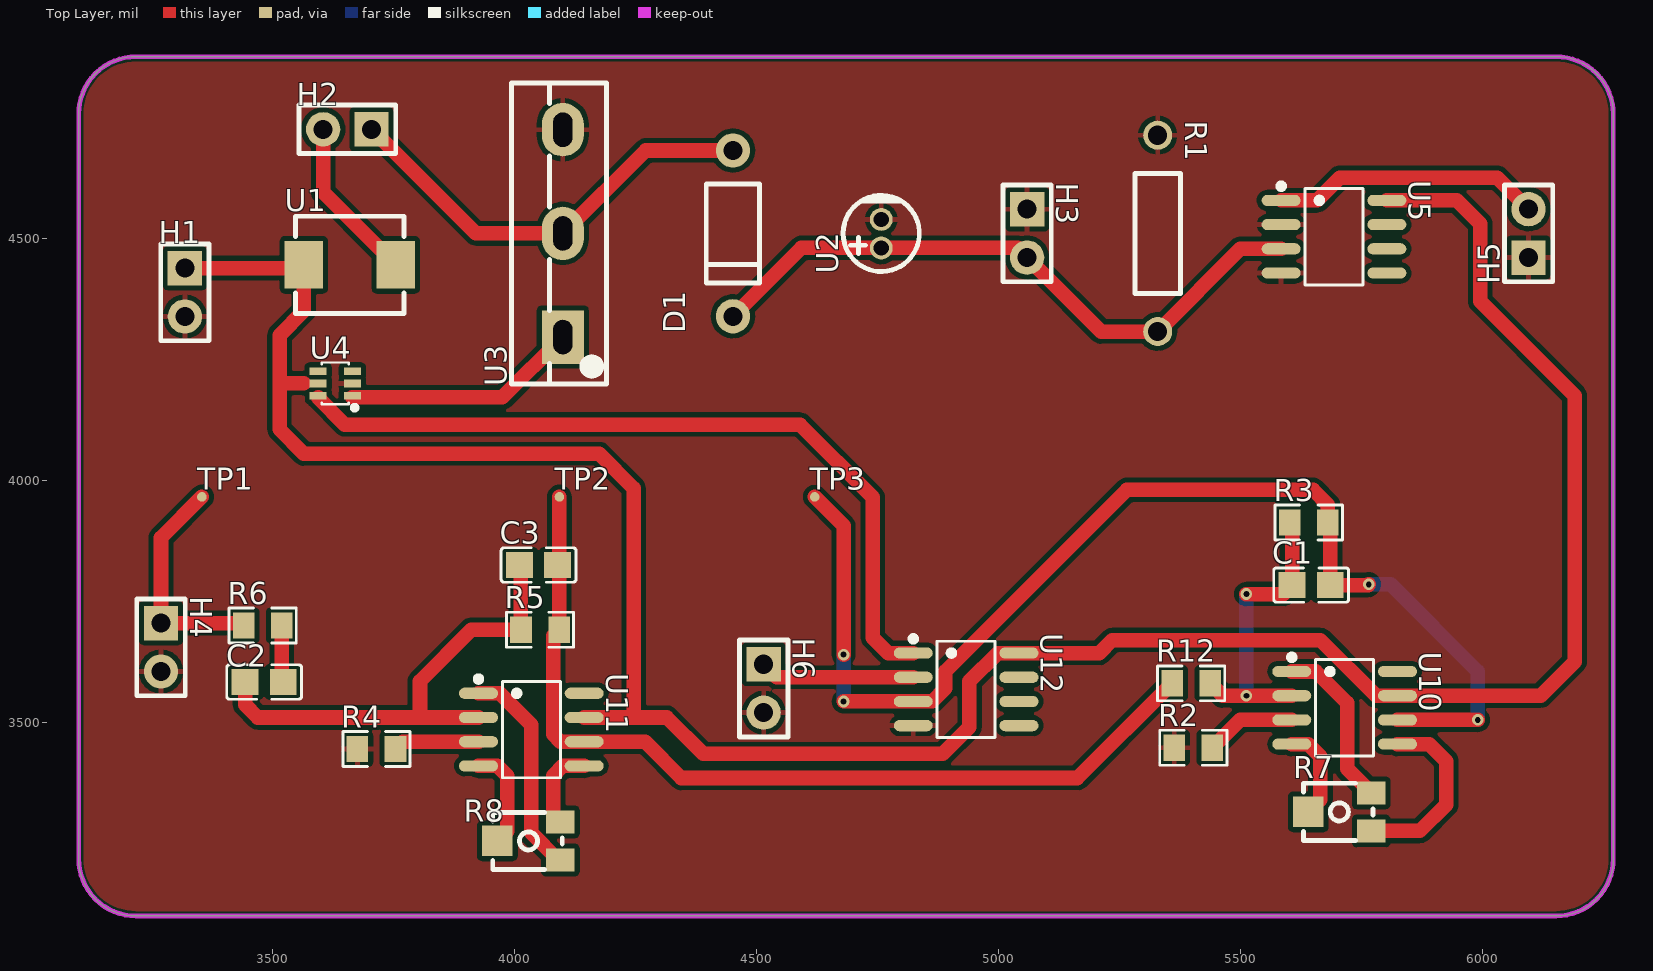
[diagram p0: Top Layer view]
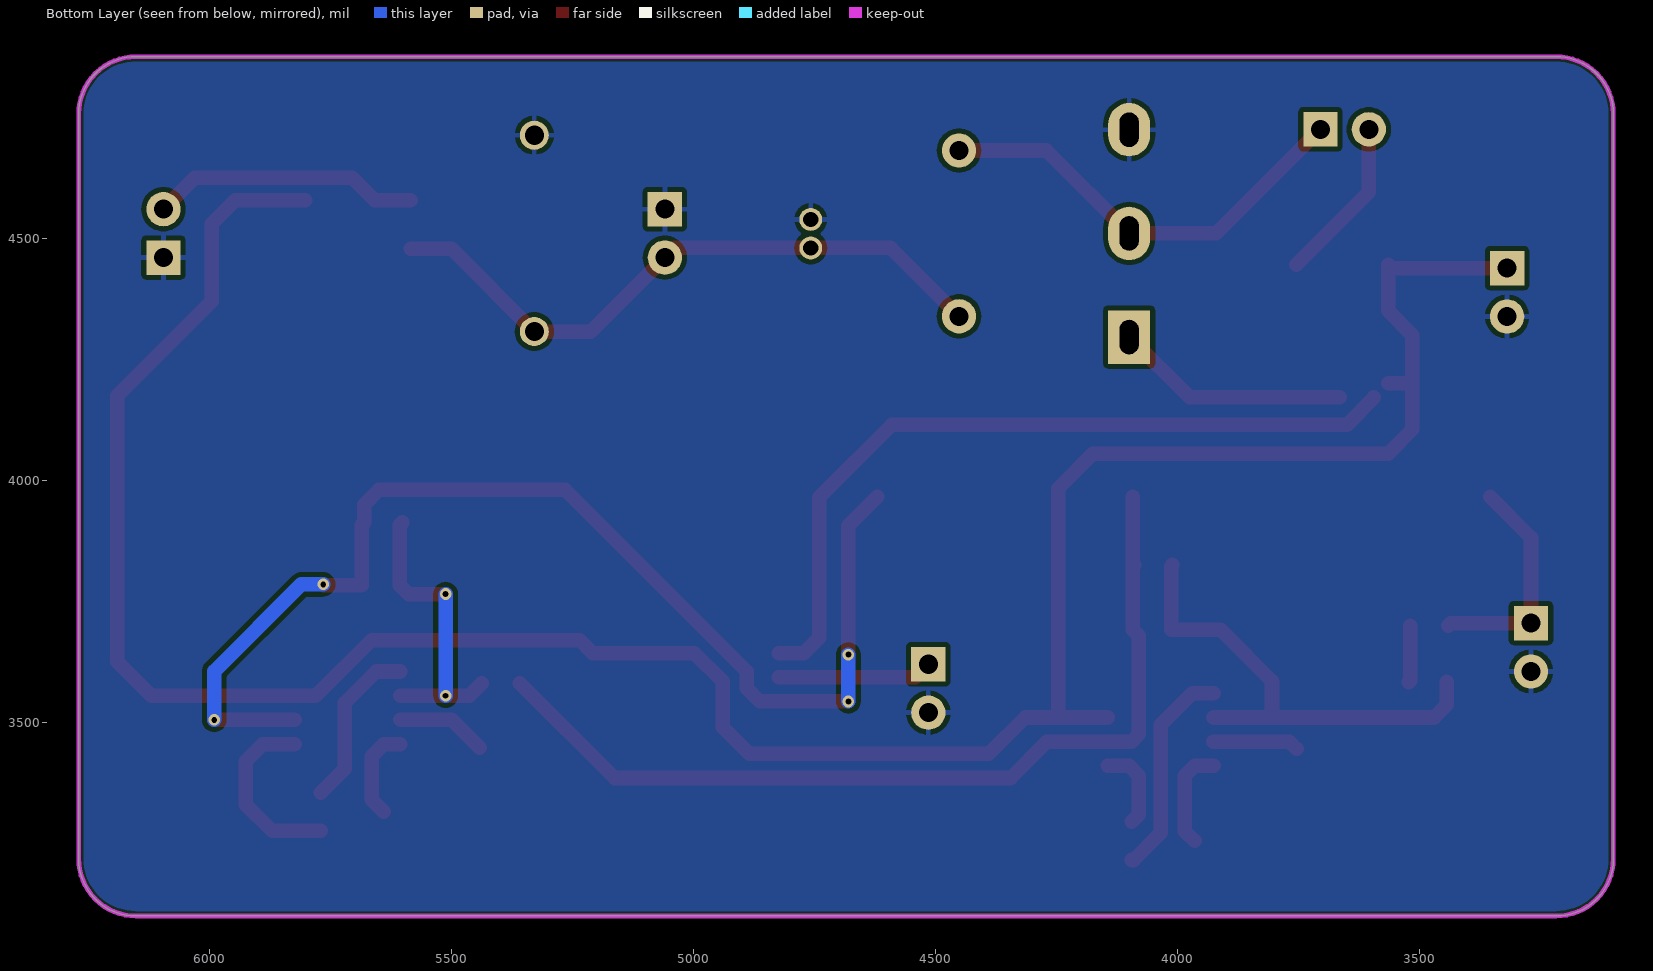
[diagram p1: Bottom Layer view, seen from below]
# Altium PCB MISC89040.pcbdoc
Units mil, origin at the board's own origin, x right, y up, seen from the top; angles counter-clockwise.
Board outline 3170 x 1775 mil, 2 copper layers (Top Layer, Bottom Layer), stack 62.206 mil thick; 30 components, 23 nets, 88 pads, 6 vias.

## Layer stack, top to bottom
Top Solder Mask Layer: solder mask 0.394, Dk 3.3
Top Layer: signal copper 1.379
Dielectric1: surface 59.449, FR4, Dk 4.5
Bottom Layer: signal copper 1.378
Bottom Solder Mask Layer: solder mask 0.394, Dk 3.3

## Board outline
3218.11,4875 ccw(c3218.11,4756.89) 3100,4756.89 3100,3218.11 ccw(c3218.11,3218.11) 3218.11,3100 6151.89,3100 ccw(c6151.89,3218.11) 6270,3218.11 6270,4756.89 ccw(c6151.89,4756.89) 6151.89,4875

## Design rules (kind name [scope] priority, off if disabled: settings)
BoardOutlineClearance copperThickness2oz_1 [All] p2 off: genericclearance=7.99 ignorepadtopadclearanceinfootprint=FALSE except(0: Arc-SplitContinuation Track-SplitContinuation SMDPad-SplitContinuation THPad-SplitContinuation Via-SplitContinuation Fill-SplitContinuation Region-SplitContinuation Poly-SplitContinuation Text-SplitContinuation Hole-SplitContinuation; 5.98: Arc-CutoutEdge Track-CutoutEdge SMDPad-CutoutEdge THPad-CutoutEdge Via-CutoutEdge Text-CutoutEdge; 6.9: Hole-OutlineEdge Hole-CutoutEdge; 10: Poly-OutlineEdge Poly-CutoutEdge; 11.81: Arc-OutlineEdge Track-OutlineEdge SMDPad-OutlineEdge THPad-OutlineEdge Via-OutlineEdge Fill-OutlineEdge Region-OutlineEdge Text-OutlineEdge Fill-CutoutEdge Region-CutoutEdge)
BoardOutlineClearance Plane_innerPlane_1 [All] p4 off: genericclearance=4.02 ignorepadtopadclearanceinfootprint=FALSE except(0: Arc-SplitContinuation Track-SplitContinuation SMDPad-SplitContinuation THPad-SplitContinuation Via-SplitContinuation Fill-SplitContinuation Region-SplitContinuation Poly-SplitContinuation Text-SplitContinuation Hole-SplitContinuation; 5.98: Arc-CutoutEdge Track-CutoutEdge SMDPad-CutoutEdge THPad-CutoutEdge Via-CutoutEdge Text-CutoutEdge; 6.9: Hole-OutlineEdge Hole-CutoutEdge; 10: Poly-OutlineEdge Poly-CutoutEdge; 11.81: Arc-OutlineEdge Track-OutlineEdge SMDPad-OutlineEdge THPad-OutlineEdge Via-OutlineEdge Fill-OutlineEdge Region-OutlineEdge Text-OutlineEdge Fill-CutoutEdge Region-CutoutEdge)
BoardOutlineClearance Copper_copperRegion_1 [All] p6 off: genericclearance=4.02 ignorepadtopadclearanceinfootprint=FALSE except(0: Arc-SplitContinuation Track-SplitContinuation SMDPad-SplitContinuation THPad-SplitContinuation Via-SplitContinuation Fill-SplitContinuation Region-SplitContinuation Poly-SplitContinuation Text-SplitContinuation Hole-SplitContinuation; 5.98: Arc-CutoutEdge Track-CutoutEdge SMDPad-CutoutEdge THPad-CutoutEdge Via-CutoutEdge Text-CutoutEdge; 6.9: Hole-OutlineEdge Hole-CutoutEdge; 10: Poly-OutlineEdge Poly-CutoutEdge; 11.81: Arc-OutlineEdge Track-OutlineEdge SMDPad-OutlineEdge THPad-OutlineEdge Via-OutlineEdge Fill-OutlineEdge Region-OutlineEdge Text-OutlineEdge Fill-CutoutEdge Region-CutoutEdge)
BoardOutlineClearance copperThickness1oz_1 [All] p8: genericclearance=4.02 ignorepadtopadclearanceinfootprint=FALSE except(0: Arc-SplitContinuation Track-SplitContinuation SMDPad-SplitContinuation THPad-SplitContinuation Via-SplitContinuation Fill-SplitContinuation Region-SplitContinuation Poly-SplitContinuation Text-SplitContinuation Hole-SplitContinuation; 5.98: Arc-CutoutEdge Track-CutoutEdge SMDPad-CutoutEdge THPad-CutoutEdge Via-CutoutEdge Text-CutoutEdge; 6.9: Hole-OutlineEdge Hole-CutoutEdge; 10: Poly-OutlineEdge Poly-CutoutEdge; 11.81: Arc-OutlineEdge Track-OutlineEdge SMDPad-OutlineEdge THPad-OutlineEdge Via-OutlineEdge Fill-OutlineEdge Region-OutlineEdge Text-OutlineEdge Fill-CutoutEdge Region-CutoutEdge)
Clearance copperThickness2oz [All] p1 off: gap=7.99 ignorepadtopadclearanceinfootprint=FALSE except(5.98: SMDPad-Track SMDPad-SMDPad THPad-Track SMDPad-THPad THPad-THPad Track-Via SMDPad-Via THPad-Via Via-Via Fill-SMDPad Region-SMDPad Fill-THPad Region-THPad Fill-Via Region-Via Fill-Fill Fill-Region Region-Region Arc-Track Arc-SMDPad Arc-THPad Arc-Via Fill-Arc Region-Arc Arc-Arc Text-Track SMDPad-Text Text-THPad Text-Via Fill-Text Region-Text Arc-Text Text-Text; 6.9: Hole-Track Hole-SMDPad Hole-THPad Hole-Via Fill-Hole Region-Hole Hole-Arc Hole-Text; 10: Poly-Track Poly-SMDPad Poly-THPad Poly-Via Poly-Fill Poly-Region Poly-Poly Poly-Arc Poly-Text Poly-Hole; 11.81: Fill-Track Region-Track)
Clearance Plane_innerPlane [All] p3 off: gap=4.02 ignorepadtopadclearanceinfootprint=FALSE except(5.98: SMDPad-Track SMDPad-SMDPad THPad-Track SMDPad-THPad THPad-THPad Track-Via SMDPad-Via THPad-Via Via-Via Fill-SMDPad Region-SMDPad Fill-THPad Region-THPad Fill-Via Region-Via Fill-Fill Fill-Region Region-Region Arc-Track Arc-SMDPad Arc-THPad Arc-Via Fill-Arc Region-Arc Arc-Arc Text-Track SMDPad-Text Text-THPad Text-Via Fill-Text Region-Text Arc-Text Text-Text; 6.9: Hole-Track Hole-SMDPad Hole-THPad Hole-Via Fill-Hole Region-Hole Hole-Arc Hole-Text; 10: Poly-Track Poly-SMDPad Poly-THPad Poly-Via Poly-Fill Poly-Region Poly-Poly Poly-Arc Poly-Text Poly-Hole; 11.81: Fill-Track Region-Track)
Clearance Copper_copperRegion [All] p5 off: gap=4.02 ignorepadtopadclearanceinfootprint=FALSE except(5.98: SMDPad-Track SMDPad-SMDPad THPad-Track SMDPad-THPad THPad-THPad Track-Via SMDPad-Via THPad-Via Via-Via Fill-SMDPad Region-SMDPad Fill-THPad Region-THPad Fill-Via Region-Via Fill-Fill Fill-Region Region-Region Arc-Track Arc-SMDPad Arc-THPad Arc-Via Fill-Arc Region-Arc Arc-Arc Text-Track SMDPad-Text Text-THPad Text-Via Fill-Text Region-Text Arc-Text Text-Text; 6.9: Hole-Track Hole-SMDPad Hole-THPad Hole-Via Fill-Hole Region-Hole Hole-Arc Hole-Text; 10: Poly-Track Poly-SMDPad Poly-THPad Poly-Via Poly-Fill Poly-Region Poly-Poly Poly-Arc Poly-Text Poly-Hole; 11.81: Fill-Track Region-Track)
Clearance copperThickness1oz [All] p7: gap=4.02 ignorepadtopadclearanceinfootprint=FALSE except(5.98: SMDPad-Track SMDPad-SMDPad THPad-Track SMDPad-THPad THPad-THPad Track-Via SMDPad-Via THPad-Via Via-Via Fill-SMDPad Region-SMDPad Fill-THPad Region-THPad Fill-Via Region-Via Fill-Fill Fill-Region Region-Region Arc-Track Arc-SMDPad Arc-THPad Arc-Via Fill-Arc Region-Arc Arc-Arc Text-Track SMDPad-Text Text-THPad Text-Via Fill-Text Region-Text Arc-Text Text-Text; 6.9: Hole-Track Hole-SMDPad Hole-THPad Hole-Via Fill-Hole Region-Hole Hole-Arc Hole-Text; 10: Poly-Track Poly-SMDPad Poly-THPad Poly-Via Poly-Fill Poly-Region Poly-Poly Poly-Arc Poly-Text Poly-Hole; 11.81: Fill-Track Region-Track)
DiffPairsRouting differentialPair [All] p1: maxlimit=6 minlimit=6 mostfreqgap=6 toplayer_minwidth=5 toplayer_prefwidth=10 toplayer_maxwidth=100 toplayer_mingap=6 toplayer_prefgap=6 toplayer_maxgap=6 bottomlayer_minwidth=5 bottomlayer_prefwidth=10 bottomlayer_maxwidth=100 bottomlayer_mingap=6 bottomlayer_prefgap=6 bottomlayer_maxgap=6 maxuncoupledlength=10
HoleToHoleClearance otherClearance [All] p1: gap=11.81 allowstackedmicrovias=TRUE
Length netLength [All] p1: minlimit=0 maxlimit=0
PasteMaskExpansion pasteMaskExpansion [All] p1: expansion=0
PlaneConnect innerPlane [All] p1: planeconnectstyle=Relief reliefexpansion=20 reliefentries=4 reliefconductorwidth=10 reliefairgap=10
PolygonConnect copperRegion [All] p1: connectstyle=Relief reliefconductorwidth=10 reliefentries=4 polygonreliefangle="90 Angle" airgapwidth=10 via.connectstyle=Relief via.reliefconductorwidth=10 via.reliefentries=4 via.polygonreliefangle="90 Angle" via.airgapwidth=10
RoutingVias viaSize [All] p1: holewidth=12.01 width=24.02 viastyle="Through Hole" minholewidth=11.81 minwidth=19.68 maxholewidth=248.03 maxwidth=393.7
SolderMaskExpansion solderMaskExpansion [IsVia] p1: expansion=-1000 istentingtop=TRUE
SolderMaskExpansion solderMaskExpansion [All] p2: expansion=2 istentingtop=FALSE
Width copperThickness2oz_2 [All] p1 off: maxlimit=100 minlimit=8 preferedwidth=10
Width copperThickness1oz_2 [All] p2: maxlimit=100 minlimit=5 preferedwidth=10

## Components (designator, comment, footprint, x,y, rotation, side; value= is the part's Value field where it differs from the comment)
C1 "100nF" C0805 5645.88,3783.59 r0 top
C2 "100nF" C0805 3483.1,3583.33 r180 top
C3 "1nF" C0805 4050,3825 r0 top
D1 "" DO_1N4007 4451.5,4510 r90 top
H1 "" HDR-TH_2P-P2.54-V-M-1 3319.36,4388.27 r270 top
H2 "" HDR-TH_2P-P2.54-V-M-1 3655,4725 r180 top
H3 "" HDR-TH_2P-P2.54-V-M-1 5059.14,4510 r270 top
H4 "" HDR-TH_2P-P2.54-V-M-1 3270,3655 r270 top
H5 "" HDR-TH_2P-P2.54-V-M-1 6095,4510 r90 top
H6 "" HDR-TH_2P-P2.54-V-M-1 4515,3570 r270 top
R1 "10kΩ" Res_1/4W 5328.9,4510 r270 top
R2 "10kΩ" R0805 5402.41,3447.47 r0 top
R3 "1MΩ" R0805 5640.88,3912.79 r0 top
R4 "10kΩ" R0805 3715,3445 r0 top
R5 "10kΩ" R0805 4052.94,3691.23 r0 top
R6 "100Ω" R0805 3480,3700 r0 top
R7 "100kΩ" RES-ADJ-SMD_VG039NCH 5705,3315 r0 top
R8 "100kΩ" RES-ADJ-SMD_VG039NCH 4030,3255 r0 top
R12 "10kΩ" R0805 5398.06,3580.66 r0 top
TP1 "" Test-Point-0.5mm 3354.36,3965.8 r0 top
TP2 "" Test-Point-0.5mm 4092.94,3965.8 r0 top
TP3 "" Test-Point-0.5mm 4620.38,3965.8 r0 top
U1 "Power inductor (SMD),CKST0502-10uH/M,10uH,±20%,3A,package 5.7mm*5.1mm*2.0mm,CENKER,RoHS" IND-SMD_L5.7-W5.1 3660,4445 r0 top
U2 "10uF" CAP-TH_BD4.0-P1.50-D0.8-FD 4757.84,4509.4 r90 top
U3 "HY5204" TO-247-3_L15.8-W5.0-P5.44-L-1 4100,4510 r90 top
U4 "SN74LVC2G04DCKR" SOT-363_L2.0-W1.3-P0.65-LS2.1-BR 3630,4200 r0 top
U5 "NE5532DR" SOIC-8_L4.9-W3.9-P1.27-LS6.0-BL 5693.07,4503.13 r270 top
U10 "UA741CDT" SOIC-8_L4.9-W3.9-P1.27-LS6.0-BL 5715,3530 r270 top
U11 "UA741CDT" SOIC-8_L4.9-W3.9-P1.27-LS6.0-BL 4035,3485 r270 top
U12 "NE5532DR" SOIC-8_L4.9-W3.9-P1.27-LS6.0-BL 4933.13,3568.13 r270 top

## Footprints (in the part's own frame and the unit in brackets; to place one, negate y for a bottom-side part, rotate by r counter-clockwise, add the part's x,y. Pads: shape width x height; smd on the part's side, far side on the other; paste and mask are expansions set on the pad)
C0805 [mm]
  rect 1.41x1.35 smd paste-100 mask+0.051: 1(-1,0) 2(1,0)
  silkscreen extent -1.96,-0.9 1.96,0.9
CAP-TH_BD4.0-P1.50-D0.8-FD [mm]
  round 1.2 hole 0.8: 1(-0.75,0) 2(0.75,0)
  silkscreen extent -1.98,-2 2.06,2
DO_1N4007 [mm]
  round 1.8 hole 1 paste+0 mask+0.051: 1(-4.35,0) 2(4.35,0)
  silkscreen extent -2.6,-1.4 2.6,1.4
HDR-TH_2P-P2.54-V-M-1 [mm]
  rect 1.8x1.8 hole 1: 1(-1.27,0)
  round 1.8 hole 1: 2(1.27,0)
  silkscreen extent -2.54,-1.27 2.54,1.27
IND-SMD_L5.7-W5.1 [mm]
  rect 2x2.5 smd paste+0 mask+0.05: 1(-2.413,0) 2(2.413,0)
  silkscreen extent -2.85,-2.55 2.85,2.55
R0805 [mm]
  rect 1.133x1.377 smd paste-100 mask+0.051: 1(-1,0) 2(1,0)
  silkscreen extent -1.76,-0.92 1.76,0.92
RES-ADJ-SMD_VG039NCH [mm]
  rect 1.5x1.2 smd: 1(1.65,-1) 3(1.65,1)
  rect 1.6x1.6 smd: 2(-1.65,0)
  silkscreen extent -1.9,-1.5 1.75,1.5
Res_1/4W [mil]
  round 60 hole 39.37 paste+0 mask+2: 1(-202.76,0) 2(202.76,0)
  silkscreen extent -124,-47 124,47
SOIC-8_L4.9-W3.9-P1.27-LS6.0-BL [mm]
  oval 0.588x2.045 smd: 1(-1.905,-2.772) 2(-0.635,-2.772) 3(0.635,-2.772) 4(1.905,-2.772) 5(1.905,2.772) 6(0.635,2.772) 7(-0.635,2.772) 8(-1.905,2.772)
  silkscreen extent -2.8,-2.92 2.53,1.52
SOT-363_L2.0-W1.3-P0.65-LS2.1-BR [mm]
  rect 0.9x0.4 smd: 1(0.9,-0.65) 2(0.9,0) 3(0.9,0.65) 4(-0.9,0.65) 5(-0.9,0) 6(-0.9,-0.65)
  silkscreen extent -0.7,-1.4 1.14,1.1
Test-Point-0.5mm [mm]
  round 0.5 smd: 1(0,0)
TO-247-3_L15.8-W5.0-P5.44-L-1 [mm]
  rect 2.8x2.2 hole 1 slot 1.8 at 0 deg paste+0 mask+0.05: 1(-5.44,0)
  oval 2.8x2.2 hole 1 slot 1.8 at 0 deg paste+0 mask+0.05: 2(0,0) 3(5.44,0)
  silkscreen extent -7.9,-2.3 7.9,2.7

## Via types
v1: diameter 24, hole 12, Top Layer to Bottom Layer, 5 vias
v2: diameter 24.02, hole 12, Top Layer to Bottom Layer, 1 vias

## Nets (pads, with @x,y where several pads share a name; then routed paths per layer and width w, separated by ;. In a path a pad name is that pad's centre, name@x,y a point inside that pad or via, vN(x,y) a via of type N, cw(c..) or ccw(c..) an arc to the next point about the centre after c; other vN are vias at no path point)
$1N178: H2.2 U1.2 | length 342.1
  Top Layer w30: H2.2 3605,4595 U1.2
$1N206: D1.2 H2.1 U3.2 | length 906.5
  Top Layer w30: H2.1 3920,4510 U3.2 4271.26,4681.26 D1.2
$1N266: D1.1 H3.2 R1.2 U2.1 U5.3 | length 1333.2
  Top Layer w30: D1.1 4592.63,4479.87 U2.1 5039.27,4479.87 H3.2 5211.9,4307.24 R1.2 5499.79,4478.13 U5.3
$1N648: U3.1 U4.1 | length 486.2
  Top Layer w30: U4.1@3665.43,4171.15 3975.32,4171.15 U3.1
$1N1018: H4.1 R6.1 TP1.1 | length 468.4
  Top Layer w30: TP1.1 3270,3881.44 H4.1 3435.63,3705 R6.1
$1N3426: R7.3 U10.1 | length 347.4
  Top Layer w30: U10.1 5655,3605 5720,3540 5720,3404.33 R7.3
$1N3427: R7.1 U10.5 | length 382.9
  Top Layer w30: R7.1 5870.63,3275.63 5925,3330 5925,3420 5890,3455 U10.5
$1N3428: R2.2 U10.3 | length 187.9
  Top Layer w30: R2.2 5499.32,3505 U10.3
$1N3429: C1.1 R3.1 R12.2 U10.2 | length 622.5
  Top Layer w30: R12.2 5463.09,3555 v2(5512.02,3555) U10.2 ; v1(5512.02,3765) 5587.92,3765 C1.1 5606.51,3907.79 R3.1
  Bottom Layer w30: v2(5512.02,3555) v1(5512.02,3765)
$1N3432: C1.2 R3.2 TP3.1 U10.6 U12.3 | length 2475.6
  Top Layer w30: TP3.1 4680,3906.17 v1(4680,3640) ; v1(4680,3543.13) U12.3 4863.13,3543.13 4890,3570 4890,3605 5265,3980 5650,3980 5680.25,3949.75 R3.2 5685.25,3907.79 C1.2 5763.59,3783.59 v1(5765,3785) ; U10.6 v1(5990,3505)
  Bottom Layer w30: v1(4680,3543.13) v1(4680,3640) ; v1(5765,3785) 5810,3785 5990,3605 v1(5990,3505)
$1N3433: C3.2 R5.2 R12.1 TP2.1 U11.6 | length 1895.6
  Top Layer w30: TP2.1 4092.94,3828.57 C3.2 4092.31,3822.06 R5.2 4080,3678.92 4080,3475 4095,3460 U11.6 4270,3460 4345,3385 5163.02,3385 R12.1
$1N3435: C2.1 R6.2 | length 118
  Top Layer w30: R6.2 3519.37,3586.43 C2.1
$1N3436: R4.2 U11.3 | length 177.7
  Top Layer w30: R4.2 3769.37,3460 U11.3
$1N3437: R8.1 U11.1 | length 442.7
  Top Layer w30: U11.1 3970,3560 4035,3495 4035,3271.51 4090.88,3215.63 R8.1
$1N3439: R8.3 U11.5 | length 174.3
  Top Layer w30: R8.3 4080,3309.33 4080,3390 4100,3410 U11.5
$1N3440: C2.2 C3.1 R5.1 U11.2 | length 1006.1
  Top Layer w30: C2.2 3443.73,3536.27 3470,3510 3796.55,3510 ; U11.2 3796.55,3510 ; C3.1 4013.57,3822.06 R5.1 3911.23,3691.23 3805,3585 3805,3518.45 3796.55,3510
$1N3876: H6.1 U12.2 | length 320.1
  Top Layer w30: H6.1 4541.87,3593.13 U12.2
-9V: R8.2 U11.4 | length 210.7
  Top Layer w30: U11.4 3965,3410 3985,3390 3985,3274.96 R8.2
-VCC: R7.2 U10.4 | length 194.8
  Top Layer w30: U10.4 5640,3455 5665,3430 5665,3339.96 R7.2
GND: H1.2 H3.1 H4.2 H5.1 H6.2 R1.1 R2.1 R4.1 U2.2 U3.3 U4.2 U5.2 U5.4 U12.4
VC: U4.6 U12.1 | length 1618.4
  Top Layer w30: U4.6@3594.57,4171.15 3594.57,4170.43 3650,4115 4590,4115 4740,3965 4740,3675 4771.87,3643.13 U12.1
VCC: H1.1 U1.1 U4.5 U5.8 U10.7 U11.7 U12.8 | length 5419.7
  Top Layer w30: H1.1 3558.27,4438.27 U1.1 3565,4350 3515,4300 3515,4200.49 ; 3564.89,4200 3564.4,4200.49 3515,4200.49 ; U11.7 4246.89,3510 ; U5.8 5946.87,4578.13 5995,4530 5995,4370 6190,4175 6190,3625 6120,3555 U10.7 5780,3555 5665,3670 5235,3670 5208.13,3643.13 U12.8 4998.13,3643.13 4940,3585 4940,3490 4885,3435 4390,3435 4315,3510 4246.89,3510 ; 3515,4200.49 3515,4105 3565,4055 4175,4055 4246.89,3983.11 4246.89,3510
VOUT: H5.2 U5.1 | length 557.4
  Top Layer w30: U5.1 5658.13,4578.13 5705,4625 6030,4625 H5.2
pads on no net: U4.3 U4.4 U5.5 U5.6 U5.7 U10.8 U11.8 U12.5 U12.6 U12.7

## Polygon pours and split planes (outlines as drawn)
GND on Top Layer (solid, remove dead copper, pour order 0): 3000,5015 3000,3000 6400,3000 6400,5015
GND on Bottom Layer (solid, remove dead copper, pour order 2): 3055,4995 3055,3025 6390,3025 6390,4995

## Keep-outs
Board Outline Layer:
  the board outline again, w10